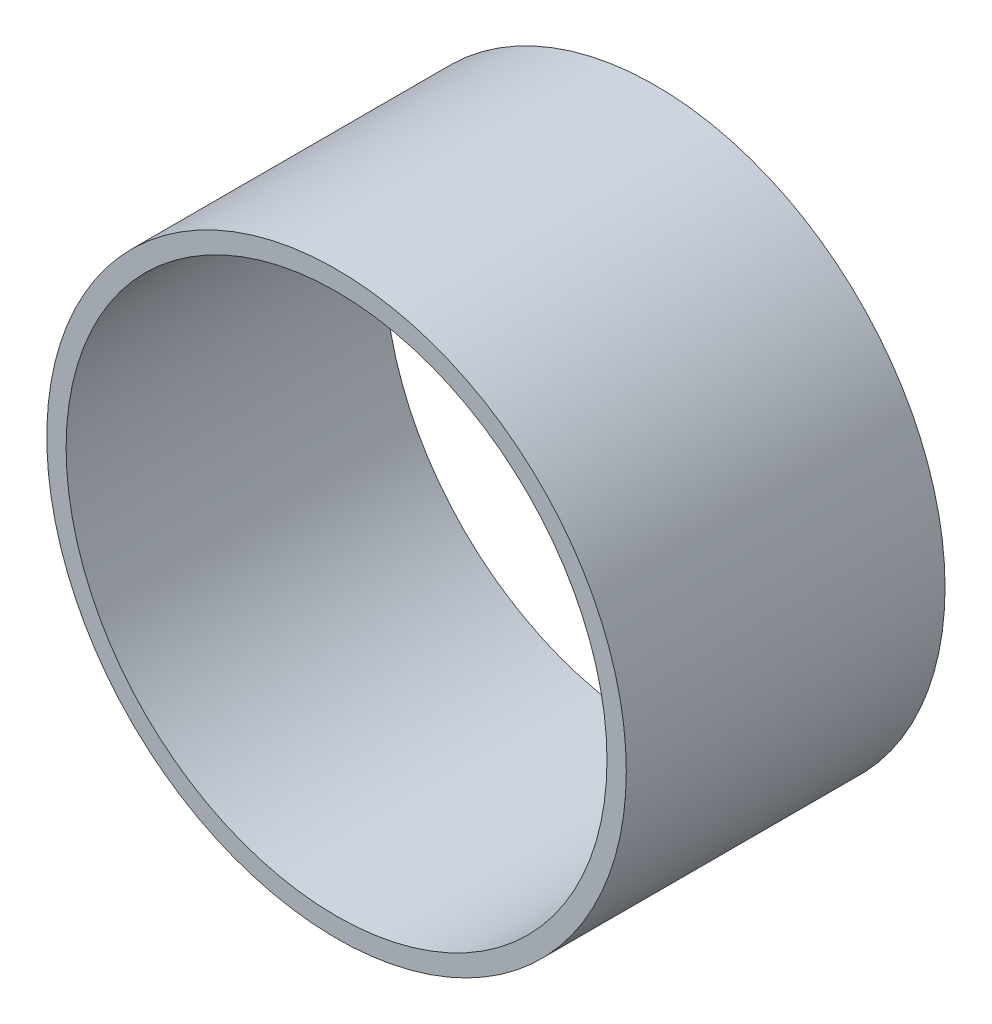
SolidWorks part; units mm, degrees
ref_plane "Front Plane" through (0, 0, 0) normal (0, 0, 1) x (1, 0, 0)
ref_plane "Top Plane" through (0, 0, 0) normal (0, 1, 0) x (1, 0, 0)
ref_plane "Right Plane" through (0, 0, 0) normal (1, 0, 0) x (0, 0, -1)
sketch "Sketch1" plane through (0, 0, 0) normal (0, 0, 1) x (1, 0, 0)
  circle A0 centre (0, 0) radius 30
  circle A1 centre (0, 0) radius 28
extrude "Boss-Extrude1" add sketch "Sketch1" along normal blind 33
